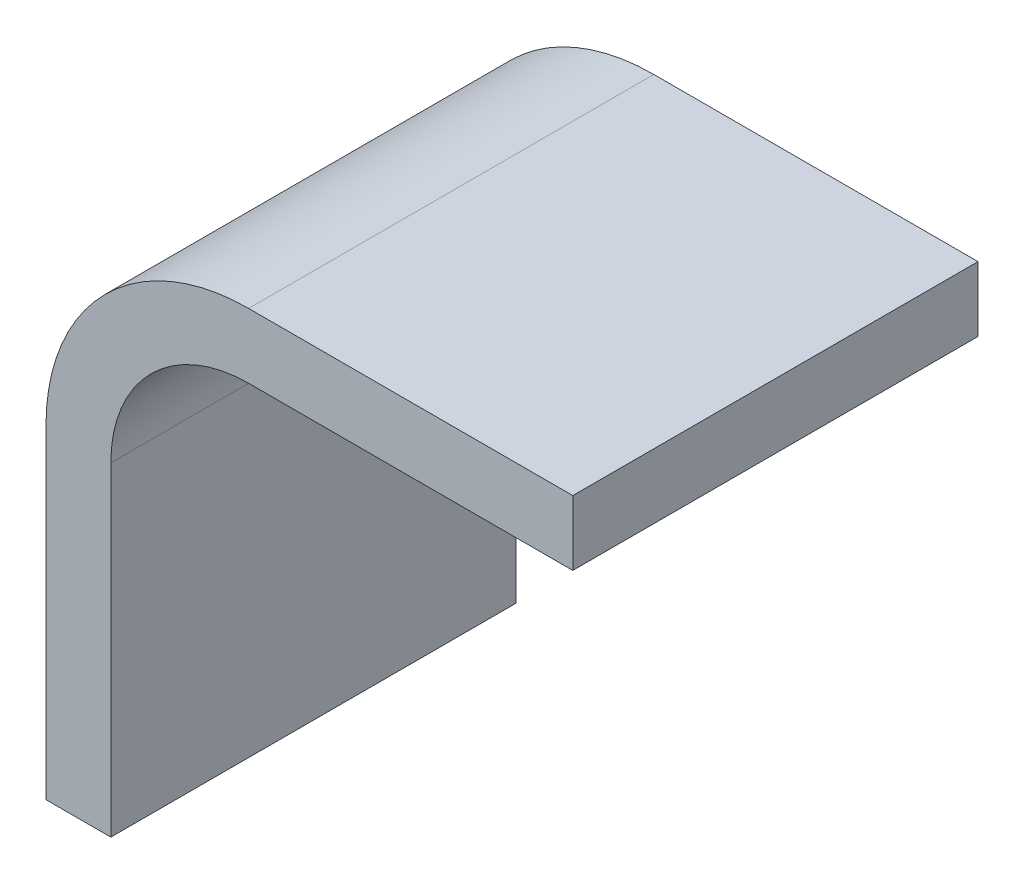
SolidWorks part; units mm, degrees
material "Plain Carbon Steel"
ref_plane "Front Plane" through (0, 0, 0) normal (0, 0, 1) x (1, 0, 0)
ref_plane "Top Plane" through (0, 0, 0) normal (0, 1, 0) x (1, 0, 0)
ref_plane "Right Plane" through (0, 0, 0) normal (1, 0, 0) x (0, 0, -1)
sketch "Sketch1" plane through (0, 0, 0) normal (0, 0, 1) x (1, 0, 0)
  line L0 (50, 0) -> (130, 0)
  line L1 (0, -50) -> (0, -130)
  arc A0 (50, 0) -> (0, -50) centre (50, -50) ccw
  point P6 (0, 0)
  dimension "D3" = 50
  dimension "D1" = 130
  dimension "D2" = 130
extrude "Extrude-Thin1" add sketch "Sketch1" along normal blind 100 thin
